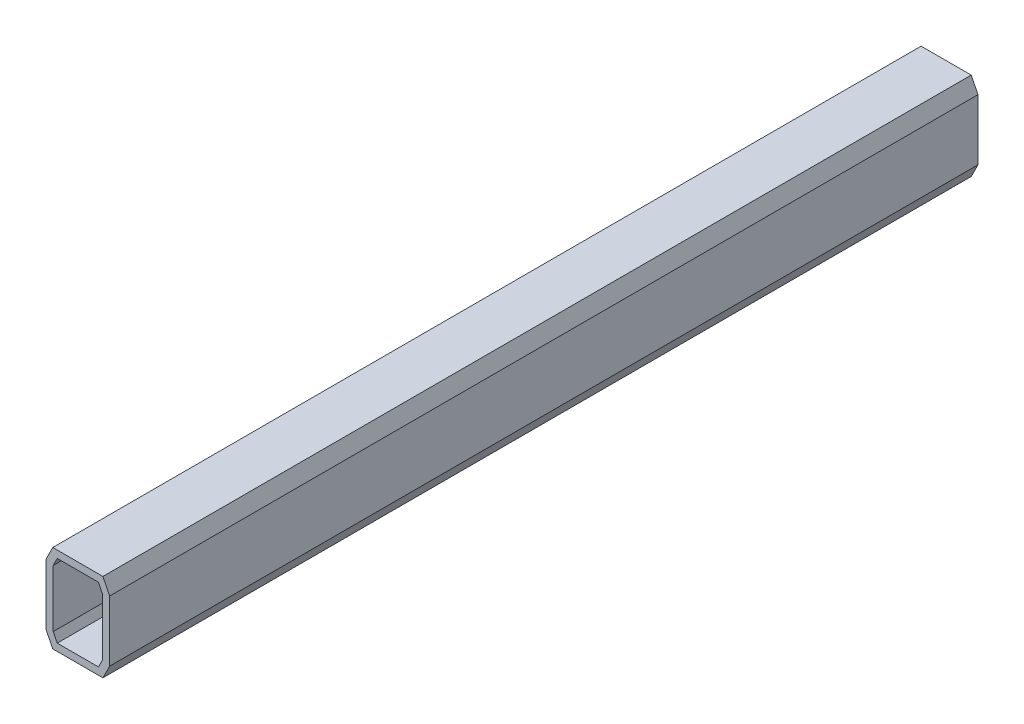
from build123d import *

# Parameters (mm, degrees)
BOSS_EXTRUDE1_DEPTH = 600


with BuildPart() as part:
    # Sketch1 → Boss-Extrude1 (new body)
    with BuildSketch(Plane.XY):
        Polygon((-17.319660113, 136.5), (17.319660113, 136.5), (22, 127.139320225), (22, 85.160679775), (17.319660113, 75.8), (-17.319660113, 75.8), (-22, 85.160679775), (-22, 127.139320225), align=None)
        Polygon((-14.229490169, 131.5), (14.229490169, 131.5), (17, 125.958980338), (17, 86.341019662), (14.229490169, 80.8), (-14.229490169, 80.8), (-17, 86.341019662), (-17, 125.958980338), align=None, mode=Mode.SUBTRACT)
    extrude(amount=BOSS_EXTRUDE1_DEPTH)


solid = part.part
